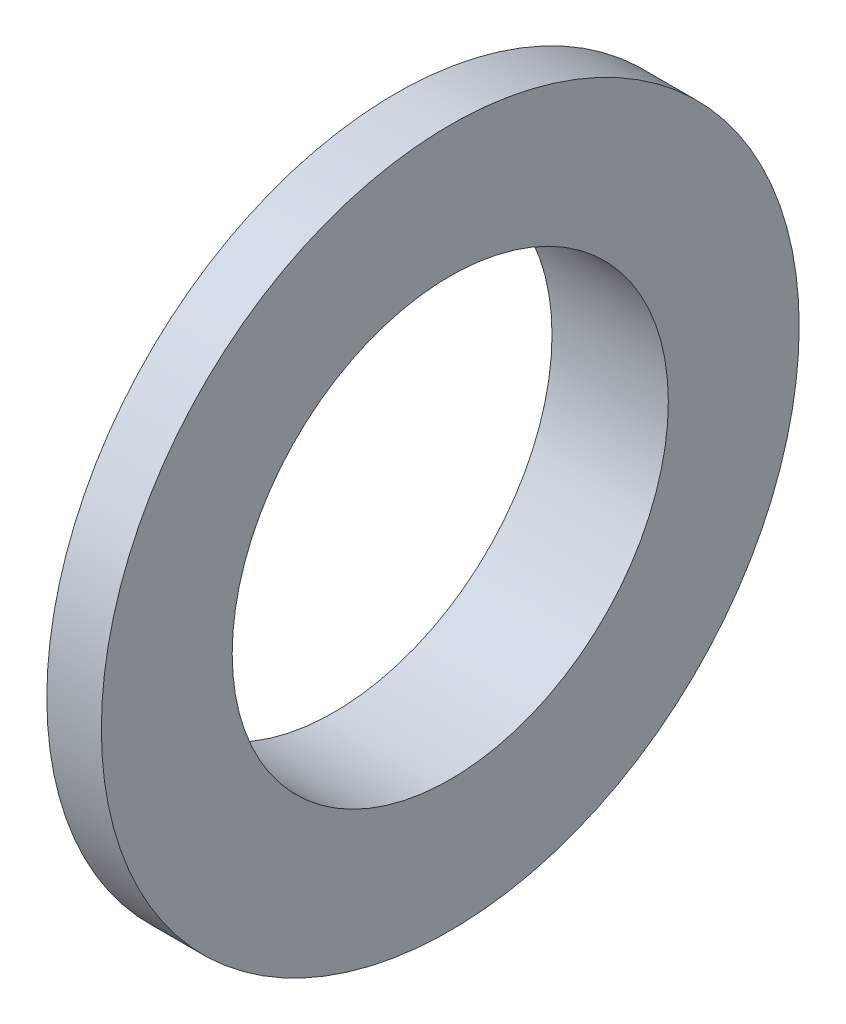
SolidWorks part; units mm, degrees
material "灰铸铁 HT150 "
ref_plane "Front Plane" through (0, 0, 0) normal (0, 0, 1) x (1, 0, 0)
ref_plane "Top Plane" through (0, 0, 0) normal (0, 1, 0) x (1, 0, 0)
ref_plane "Right Plane" through (0, 0, 0) normal (1, 0, 0) x (0, 0, -1)
sketch "Sketch1" plane through (0, 0, 0) normal (0, 0, 1) x (1, 0, 0)
  line L0 (0, 0) -> (243.7316, 0) construction
  line L1 (0, 120) -> (0, 140)
  line L2 (0, 140) -> (48, 140)
  line L4 (34, 192) -> (64, 192)
  line L5 (64, 192) -> (64, 120)
  line L6 (64, 120) -> (0, 120)
  line L11 (34, 180) -> (34, 192)
  line L12 (34, 180) -> (48, 180)
  line L13 (34, 166) -> (48, 166)
  line L14 (48, 180) -> (48, 166)
  line L15 (34, 154) -> (34, 166)
  line L16 (34, 154) -> (48, 154)
  line L18 (48, 154) -> (48, 140)
  dimension "D1" = 120
  dimension "D2" = 140
  dimension "D3" = 192
  dimension "D4" = 64
  dimension "D5" = 30
  dimension "D6" = 14
  dimension "D7" = 154
  dimension "D8" = 166
  dimension "D9" = 180
revolve "Revolve1" add sketch "Sketch1" angle 360 about L0
